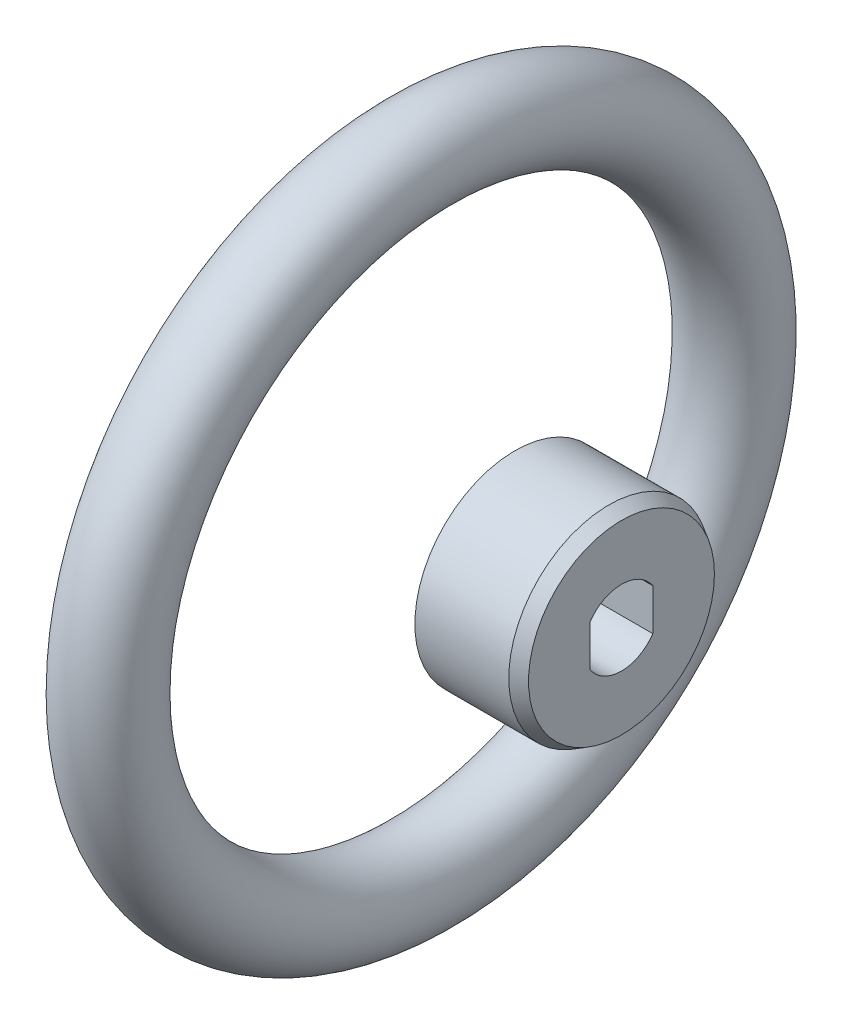
from build123d import *

# Parameters (mm, degrees)
SKETCH1_R           = 7
SKETCH3_R           = 16
BOSS_EXTRUDE1_DEPTH = 17
CHAMFER1_SIZE       = 2
CHAMFER1_SIZE2      = 1.154700538
CUT_EXTRUDE1_DEPTH  = 128.35383795


with BuildPart() as part:
    # Sweep1: sweep along a path in Sketch2
    with BuildLine(Plane(origin=(0, 0, 0), x_dir=(0, 0, -1), z_dir=(1, 0, 0))) as sweep1_path:
        CenterArc((0, -50), 50, 0, 360)
    # Sketch1 → Sweep1 (sweep)
    with BuildSketch(Plane.XY):
        Circle(SKETCH1_R)
    sweep(path=sweep1_path.line)


with BuildPart() as body_2:
    # Sketch3 → Boss-Extrude1 (new body)
    with BuildSketch(Plane(origin=(32, 0, 0), x_dir=(0, 0, -1), z_dir=(1, 0, 0))):
        with Locations((0, -50)):
            Circle(SKETCH3_R)
    extrude(amount=-BOSS_EXTRUDE1_DEPTH)

    # Chamfer1
    chamfer1_edges = [body_2.edges().sort_by_distance(p)[0] for p in [
        (32, -50, 16),
    ]]
    chamfer1_side = [body_2.faces().sort_by_distance(p)[0] for p in [
        (23.5, -50, 16),
    ]]
    chamfer(chamfer1_edges, length=CHAMFER1_SIZE, length2=CHAMFER1_SIZE2, reference=chamfer1_side[0])

    # Sketch6 → Cut-Extrude1 (cut, through all)
    with BuildSketch(Plane(origin=(32, 0, 0), x_dir=(0, 0, -1), z_dir=(1, 0, 0))):
        with BuildLine():
            Line((-5, -46.68337521), (-5, -53.31662479))
            ThreePointArc((-5, -53.31662479), (0, -56), (5, -53.31662479))
            Line((5, -53.31662479), (5, -46.68337521))
            ThreePointArc((5, -46.68337521), (0, -44), (-5, -46.68337521))
        make_face()
    extrude(amount=-CUT_EXTRUDE1_DEPTH, mode=Mode.SUBTRACT)


solid = Compound([part.part, body_2.part])
